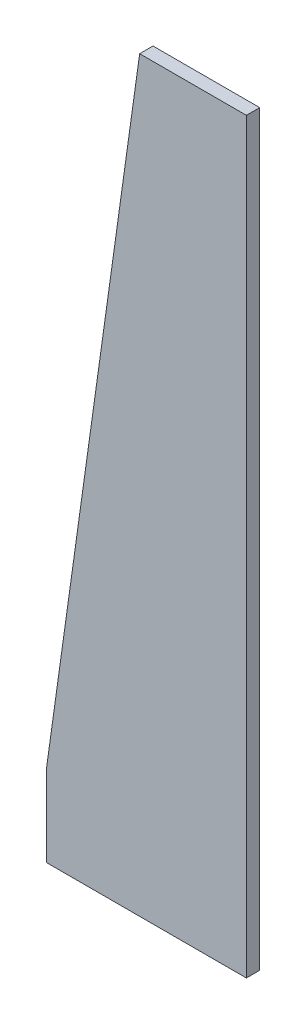
SolidWorks part; units mm, degrees
ref_plane "前视基准面" through (0, 0, 0) normal (0, 0, 1) x (1, 0, 0)
ref_plane "上视基准面" through (0, 0, 0) normal (0, 1, 0) x (1, 0, 0)
ref_plane "右视基准面" through (0, 0, 0) normal (1, 0, 0) x (0, 0, -1)
sketch "草图1" plane through (0, 0, 0) normal (0, 0, 1) x (1, 0, 0)
  line L0 (0, 0) -> (70, 0)
  line L1 (70, 0) -> (70, 280)
  line L2 (70, 280) -> (30, 280)
  line L3 (0, 0) -> (-5, 0)
  line L4 (-5, 0) -> (-5, 30)
  line L5 (-5, 30) -> (30, 280)
  line L6 (30, 280) -> (30.5332, 279.789)
extrude "凸台-拉伸3" add sketch "草图1" along normal blind 5
